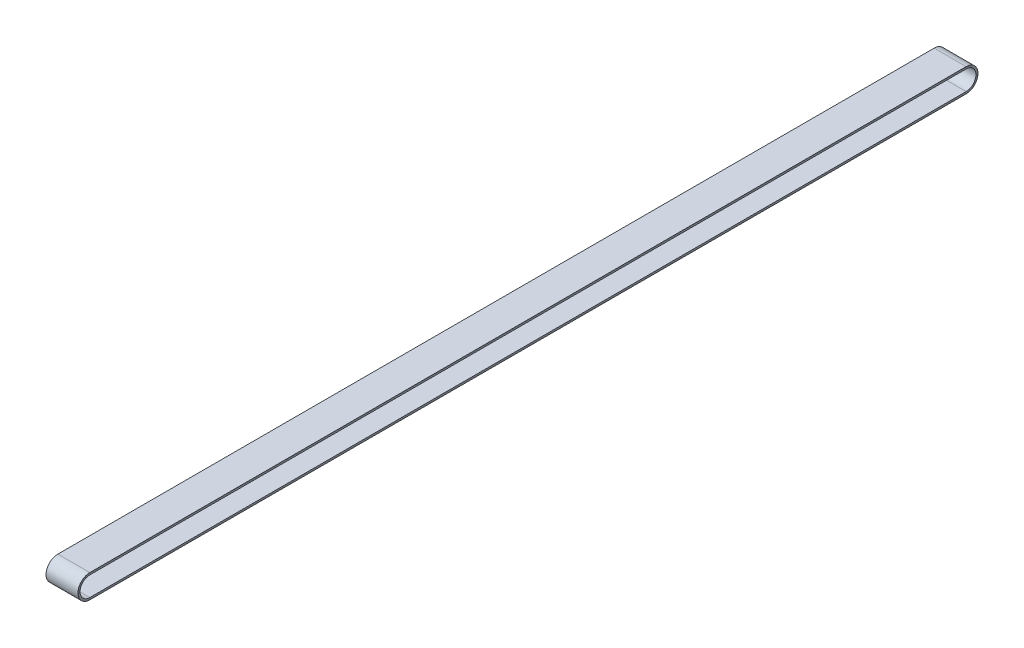
from build123d import *

# Parameters (mm, degrees)
EXTRUDE_1_DEPTH = 40
EXTRUDE_2_DEPTH = 40


with BuildPart() as part:
    # 草图1 → 拉伸-薄壁1 (new, symmetric)
    with BuildSketch(Plane(origin=(0, 0, 0), x_dir=(0, 0, -1), z_dir=(1, 0, 0))):
        with BuildLine():
            Line((2192.5, -29.575), (0, -29.575))
            ThreePointArc((0, -29.575), (-29.575, 0), (0, 29.575))
            Line((0, 29.575), (2192.5, 29.575))
            ThreePointArc((2192.5, 29.575), (2222.075, 0), (2192.5, -29.575))
        make_face()
        with BuildLine():
            Line((2192.5, -27.325), (0, -27.325))
            ThreePointArc((0, -27.325), (-27.325, 0), (0, 27.325))
            Line((0, 27.325), (2192.5, 27.325))
            ThreePointArc((2192.5, 27.325), (2219.825, 0), (2192.5, -27.325))
        make_face(mode=Mode.SUBTRACT)
    extrude(amount=EXTRUDE_1_DEPTH, both=True)


with BuildPart() as body_2:
    # 草图2 → 拉伸-薄壁2 (new, symmetric)
    with BuildSketch(Plane(origin=(0, 0, 0), x_dir=(0, 0, -1), z_dir=(1, 0, 0))):
        with BuildLine():
            Line((0, -27.325), (2192.5, -27.325))
            ThreePointArc((2192.5, -27.325), (2219.825, 0), (2192.5, 27.325))
            Line((2192.5, 27.325), (0, 27.325))
            ThreePointArc((0, 27.325), (-27.325, 0), (0, -27.325))
        make_face()
        with BuildLine():
            Line((0, -24.495), (2192.5, -24.495))
            ThreePointArc((2192.5, -24.495), (2216.995, 0), (2192.5, 24.495))
            Line((2192.5, 24.495), (0, 24.495))
            ThreePointArc((0, 24.495), (-24.495, 0), (0, -24.495))
        make_face(mode=Mode.SUBTRACT)
    extrude(amount=EXTRUDE_2_DEPTH, both=True)


solid = Compound([part.part, body_2.part])
